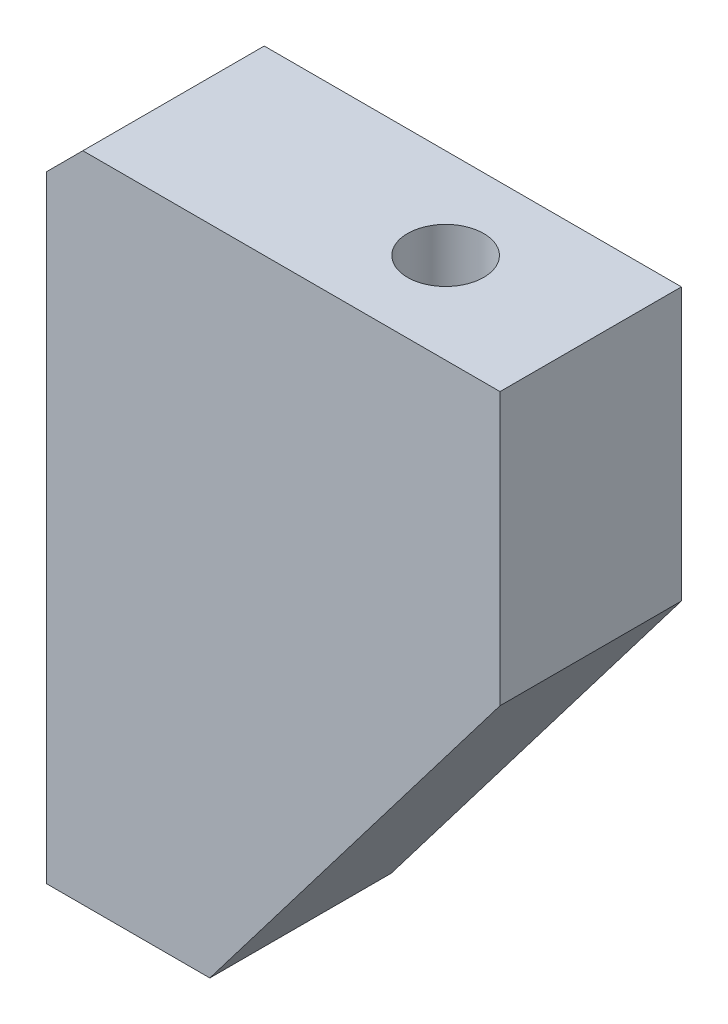
from build123d import *

# Parameters (mm, degrees)
EXTRUDE_1_DEPTH        = 10
HOLE_WIZARD_M5_2_D     = 4.2
HOLE_WIZARD_M5_2_DEPTH = 13
HOLE_WIZARD_M5_2_TIP   = 1.2618073
HOLE_WIZARD_M5_1_D     = 4.2
HOLE_WIZARD_M5_1_DEPTH = 13
HOLE_WIZARD_M5_1_TIP   = 1.2618073
CHAMFER_1_SIZE         = 2


with BuildPart() as part:
    # 草图1 → 凸台-拉伸1 (new body)
    with BuildSketch(Plane.XY):
        Polygon((-64.634074155, -10.796814071), (-39.634074155, -10.796814071), (-39.634074155, -25.796814071), (-55.634074155, -46.796814071), (-64.634074155, -46.796814071), align=None)
    extrude(amount=EXTRUDE_1_DEPTH)

    # M5 螺纹孔2
    with Locations(Plane(origin=(0, -10.796814071, 0), x_dir=(1, 0, 0), z_dir=(0, 1, 0))):
        with Locations((-47.634074155, -5)):
            Hole(HOLE_WIZARD_M5_2_D / 2, depth=HOLE_WIZARD_M5_2_DEPTH)
            with Locations((0, 0, -(HOLE_WIZARD_M5_2_DEPTH + HOLE_WIZARD_M5_2_TIP / 2))):  # 118° drill point
                Cone(0, HOLE_WIZARD_M5_2_D / 2, HOLE_WIZARD_M5_2_TIP, mode=Mode.SUBTRACT)

    # M5 螺纹孔1
    with Locations(Plane.ZY.offset(64.634074155)):
        with Locations((5, -18.796814071), (5, -38.796814071)):
            Hole(HOLE_WIZARD_M5_1_D / 2, depth=HOLE_WIZARD_M5_1_DEPTH)
            with Locations((0, 0, -(HOLE_WIZARD_M5_1_DEPTH + HOLE_WIZARD_M5_1_TIP / 2))):  # 118° drill point
                Cone(0, HOLE_WIZARD_M5_1_D / 2, HOLE_WIZARD_M5_1_TIP, mode=Mode.SUBTRACT)

    # 倒角1
    chamfer_1_edges = [part.edges().sort_by_distance(p)[0] for p in [
        (-64.634074155, -10.796814071, 5),
    ]]
    chamfer(chamfer_1_edges, length=CHAMFER_1_SIZE)


solid = part.part
